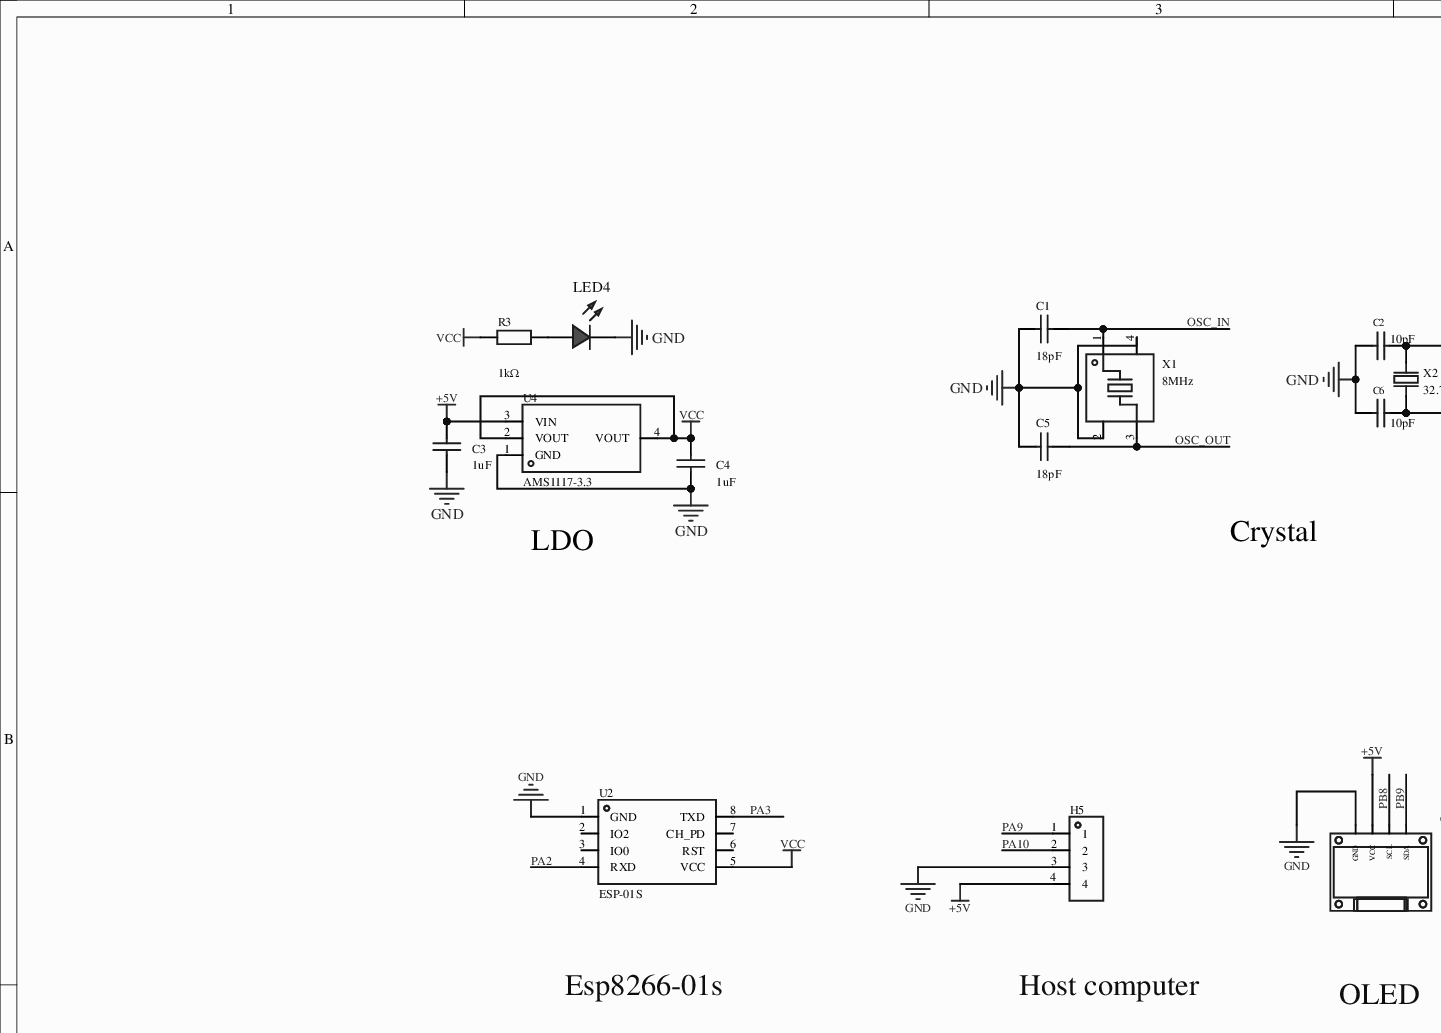
[diagram p0: MISC62726-3.schdoc, top left]
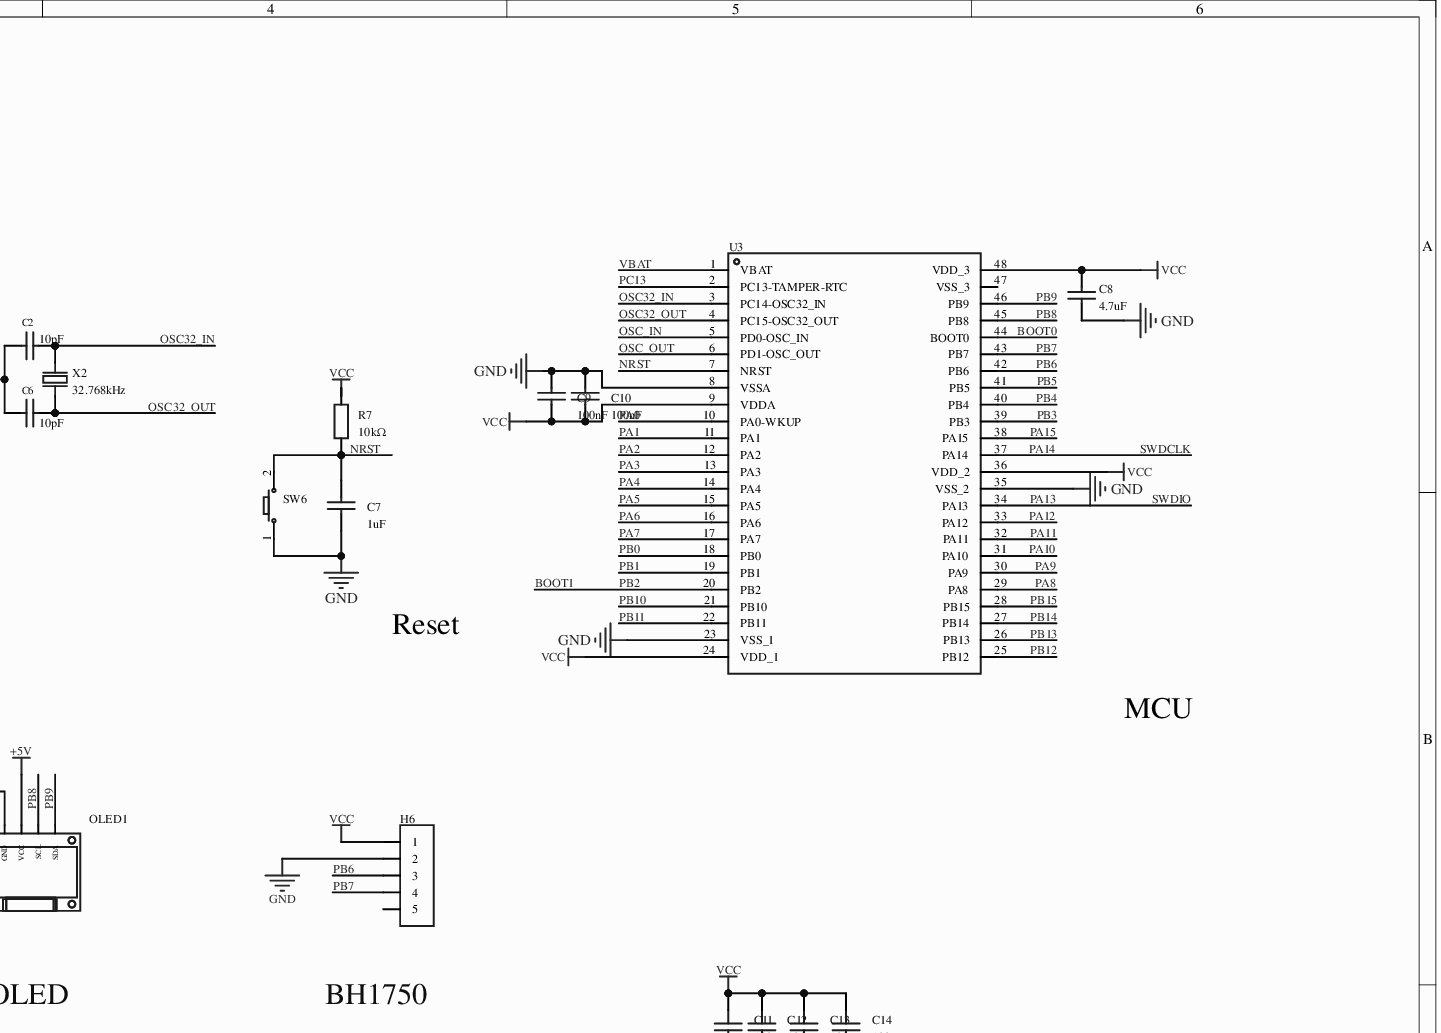
[diagram p1: MISC62726-3.schdoc, top right]
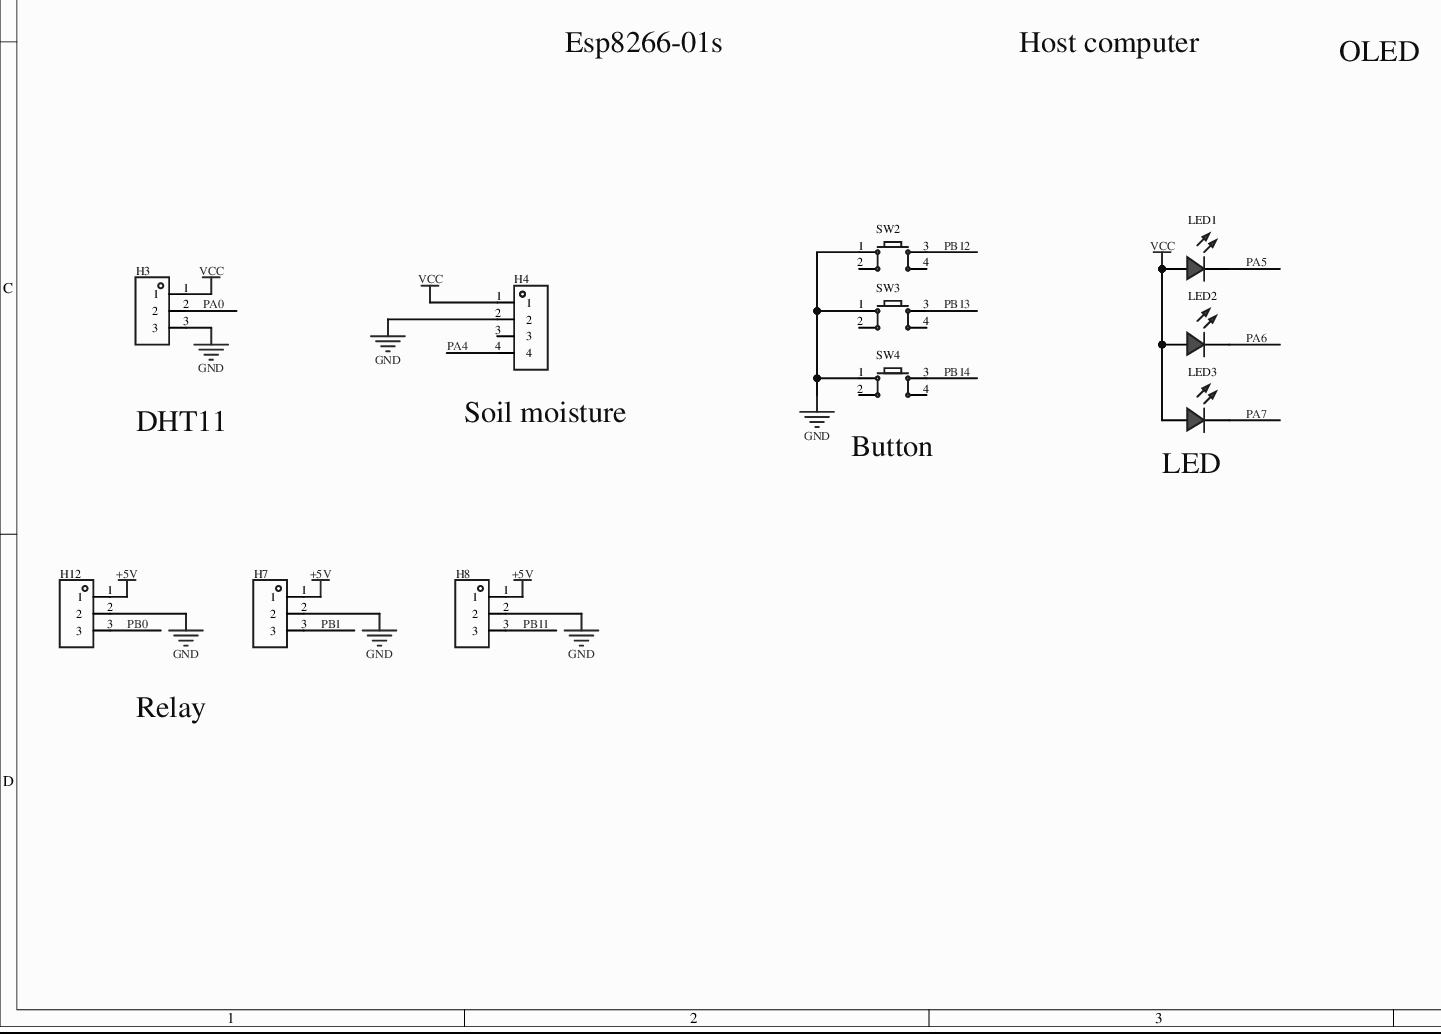
[diagram p2: MISC62726-3.schdoc, bottom left]
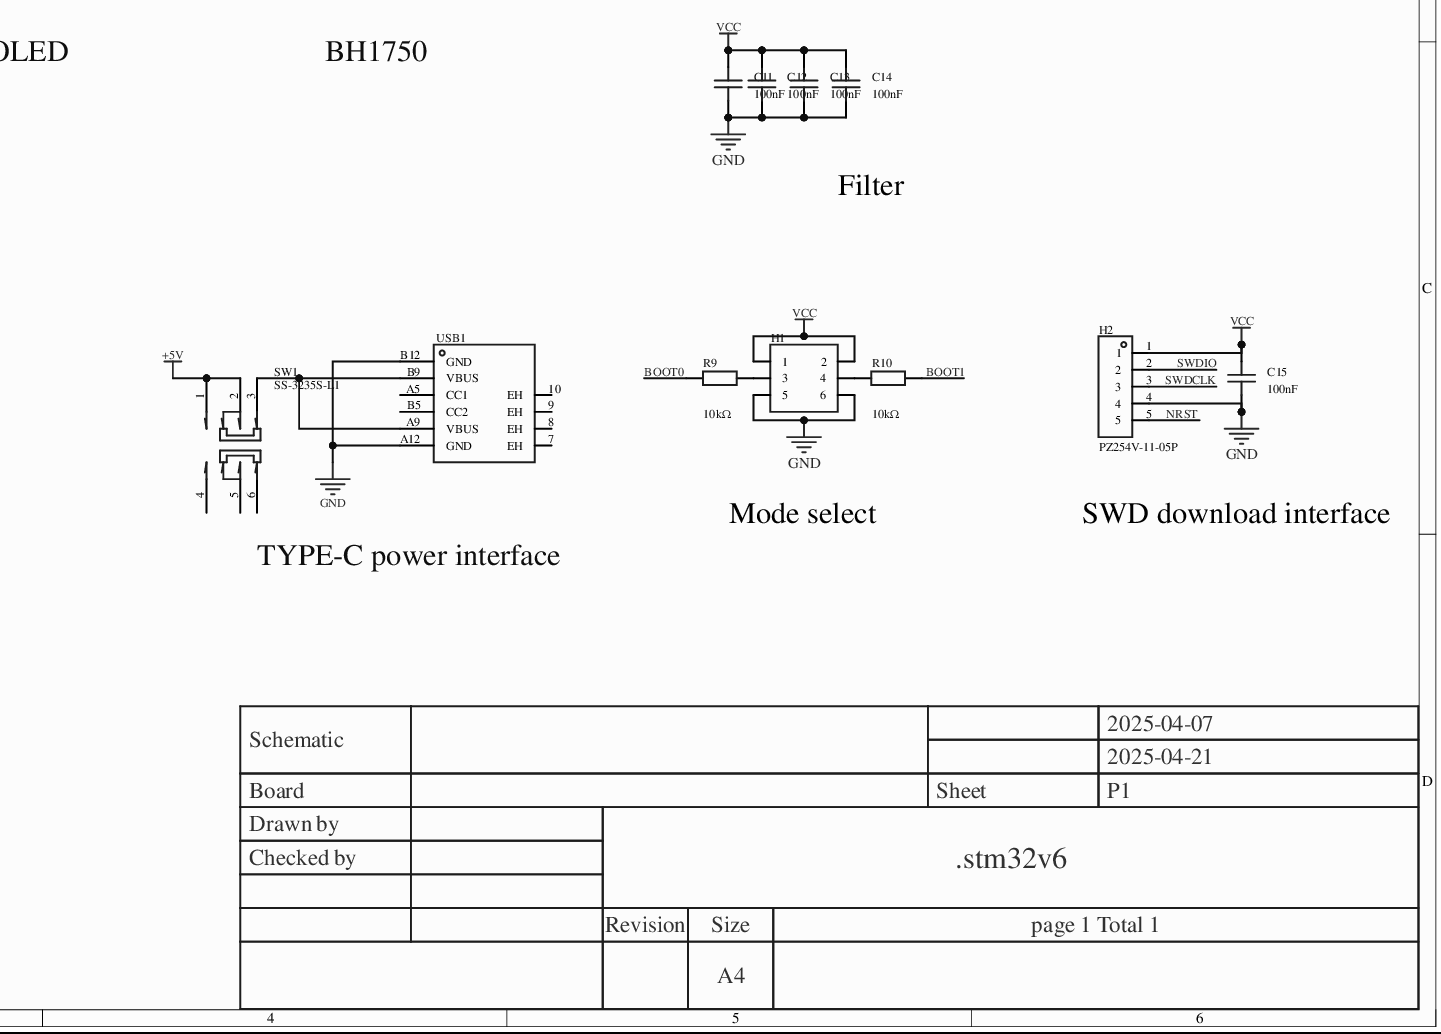
[diagram p3: MISC62726-3.schdoc, bottom right]
# Altium project MISC62726-2.PrjPcb
1 sheet, 44 parts. Net scope: global (net labels, ports and power ports of the same name join across sheets).
Board file: MISC62726.pcbdoc

## Sheet MISC62726-3.schdoc
size 420 x 297 mm; Version: V1.0; @Project Name: MISC62726; @Page Count: 1; @Update Date: 2026-04-13; @Create Date: 2026-04-13; @Schematic Name: MISC62726; @Page No: 1; @Create Time: 23:22:16; @Update Time: 17:32:40; @Board Name: MISC62726

### Parts
C1  18pF  [C0805]
C2  10pF  [C0805]
C3  1uF  [C0805]
C4  1uF  [C0805]
C5  18pF  [C0805]
C6  10pF  [C0805]
C7  1uF  [C0805]
C8  4.7uF  [C0805]
C9  100nF  [C0805]
C10  100nF  [C0805]
C11  100nF  [C0805]
C12  100nF  [C0805]
C13  100nF  [C0805]
C14  100nF  [C0805]
C15  100nF  [C0805]
H1  (no value)  [HDR-TH_6P-P2.54-V-R2-C3-S2.54_A2541WV-2X3P]
H2  PZ254V-11-05P  [HDR-TH_5P-P2.54-V-M]
H3  (no value)  [HDR-TH_3P-P2.54-V-F]
H4  (no value)  [HDR-TH_4P-P2.54-V-F]
H5  (no value)  [HDR-TH_4P-P2.54-V-F]
H6  (no value)  [HDR-TH_5P-P2.54-V-F]
H7  (no value)  [HDR-TH_3P-P2.54-V-F]
H8  (no value)  [HDR-TH_3P-P2.54-V-F]
H12  (no value)  [HDR-TH_3P-P2.54-V-F]
LED1  (no value)  [LED_TH-3mm]
LED2  (no value)  [LED_TH-3mm]
LED3  (no value)  [LED_TH-3mm]
LED4  (no value)  [LED_0402]
OLED1  (no value)  [0.96OLED_4P]
R3  1kΩ  [R0805]
R7  10kΩ  [R0805]
R9  10kΩ  [R0805]
R10  10kΩ  [R0805]
SW1  SS-3235S-L1  [SW-SMD_SS-3235S-LX]
SW2  (no value)  [SW-TH_4P-L6.0-W6.0-P4.50-LS6.5]
SW3  (no value)  [SW-TH_4P-L6.0-W6.0-P4.50-LS6.5]
SW4  (no value)  [SW-TH_4P-L6.0-W6.0-P4.50-LS6.5]
SW6  (no value)  [Key_SMD_3x4x2]
U2  ESP-01S  [WIFIM-TH_ESP-01S]
U3  STM32F103C8T6  [LQFP-48_L7.0-W7.0-P0.50-LS9.0-BL]  (value not drawn)
U4  AMS1117-3.3  [SOT-223-3_L6.5-W3.4-P2.30-LS7.0-BR]
USB1  (no value)  [USB_ TYPE-C-6P]
X1  8MHz  [OSC-SMD_4P-L3.2-W2.5-BL]
X2  32.768kHz  [CRYSTAL-SMD_L3.2-W1.5-1]

### Nets
+5V: C3.2 H5.4 H7.1 H8.1 H12.1 OLED1.2(VCC) SW1.1 SW1.2 U4.3(VIN)
GND: C1.2 C2.1 C3.1 C4.1 C5.2 C6.1 C7.2 C8.1 C9.2 C10.2 C11.1 C12.1 C13.1 C14.1 C15.1 H1.5 H1.6 H2.4 H3.3 H4.2 H5.3 H6.2 H7.2 H8.2 H12.2 LED4.1(C) OLED1.1(GND) SW2.1 SW3.1 SW4.1 SW6.1 U2.1(GND) U3.8(VSSA) U3.23(VSS_1) U3.35(VSS_2) U4.1(GND) USB1.A12(GND) USB1.B12(GND) X1.2(GND) X1.4(GND)
VCC: C4.2 C8.2 C9.1 C10.1 C11.2 C12.2 C13.2 C14.2 C15.2 H1.1 H1.2 H2.1 H3.1 H4.1 H6.1 LED1.1(C) LED2.1(C) LED3.1(C) R3.1 R7.2 U2.5(VCC) U3.9(VDDA) U3.24(VDD_1) U3.36(VDD_2) U3.48(VDD_3) U4.2(VOUT) U4.4(VOUT)
BOOT0: R9.1 U3.44(BOOT0)
BOOT1: R10.2 U3.20(PB2)  [also labelled PB2]
NRST: C7.1 H2.5 R7.1 SW6.2 U3.7(NRST)
OSC32_IN: C2.2 U3.3(PC14-OSC32_IN) X2.2
OSC32_OUT: C6.2 U3.4(PC15-OSC32_OUT) X2.1
OSC_IN: C1.1 U3.5(PD0-OSC_IN) X1.1
OSC_OUT: C5.1 U3.6(PD1-OSC_OUT) X1.3
PA0: H3.2 U3.10(PA0-WKUP)
PA1: U3.11(PA1)
PA2: U2.4(RXD) U3.12(PA2)
PA3: U2.8(TXD) U3.13(PA3)
PA4: H4.4 U3.14(PA4)
PA5: LED1.2(A) U3.15(PA5)
PA6: LED2.2(A) U3.16(PA6)
PA7: LED3.2(A) U3.17(PA7)
PA8: U3.29(PA8)
PA9: H5.1 U3.30(PA9)
PA10: H5.2 U3.31(PA10)
PA11: U3.32(PA11)
PA12: U3.33(PA12)
PA13: H2.2 U3.34(PA13)  [also labelled SWDIO]
PA14: H2.3 U3.37(PA14)  [also labelled SWDCLK]
PA15: U3.38(PA15)
PB0: H12.3 U3.18(PB0)
PB1: H7.3 U3.19(PB1)
PB3: U3.39(PB3)
PB4: U3.40(PB4)
PB5: U3.41(PB5)
PB6: H6.3 U3.42(PB6)
PB7: H6.4 U3.43(PB7)
PB8: OLED1.3(SCL) U3.45(PB8)
PB9: OLED1.4(SDA) U3.46(PB9)
PB10: U3.21(PB10)
PB11: H8.3 U3.22(PB11)
PB12: SW2.3 U3.25(PB12)
PB13: SW3.3 U3.26(PB13)
PB14: SW4.3 U3.27(PB14)
PB15: U3.28(PB15)
PC13: U3.2(PC13-TAMPER-RTC)
VBAT: U3.1(VBAT)
NetH1_3: H1.3 R9.2
NetH1_4: H1.4 R10.1
NetLED4_2: LED4.2(A) R3.2
NetSW1_3: SW1.3 USB1.A9(VBUS) USB1.B9(VBUS)

Not connected (* = marked no-connect by the designer): H4 3; H6 5; SW1 4 5 6; SW2 2 4; SW3 2 4; SW4 2 4; U2 2(IO2)* 3(IO0)* 6(RST)* 7(CH_PD)*; U3 47(VSS_3); USB1 7(EH) 8(EH) 9(EH) 10(EH) A5(CC1) B5(CC2)

### Notes on the sheet
- LDO
- Crystal
- Reset
- MCU
- Esp8266-01s
- Host computer
- OLED
- BH1750
- Filter
- DHT11
- (near H4) Soil moisture
- (near SW4) Button
- (near LED3) LED
- Mode select
- SWD download interface
- TYPE-C power interface
- Relay
- 2025-04-07
- Schematic
- Board
- Sheet
- 2025-04-21
- P1
- Drawn by
- Checked by
- .stm32v6
- Revision
- Size
- A4
- page 1 Total 1

### Library data of the parts
C1 C5 = FCC0603N180J500CT: Capacitance:18pF;Tolerance:±5%;Rated voltage:50V;Temperature coefficient:C0G;; Manufacturer: FOJAN(富捷); Symbol: 0402CG180J500NT; 3D Model: ac125912035d415993ca9572d50418b1; 3D Model Transform: 62.992,31.496,0,0,0,0,0,0,0; Tolerance: ±5%; Voltage Rating: 50V; Temperature Coefficient: C0G; AddInBom: yes; ModelName: C0603_L1.6-W0.8-H0.8; Device: FCC0603N180J500CT; Value: 18pF; LCSC Part Name: 18pF ±5% 50V; Supplier Footprint: 0603; Datasheet: https://atta.szlcsc.com/upload/public/pdf/source/20220818/0EB3B7FB2F5648AC16609637FBA7DABE.pdf; Supplier: LCSC; Manufacturer Part: FCC0603N180J500CT; Supplier Part: C5137620; JLCPCB Part Class: Extended Part; ConvertToPcb: yes; FootprintName: C0805
C2 C6 = CL10C100JB8NNNC: Capacitance:10pF;Tolerance:±5%;Rated voltage:50V;Temperature coefficient:C0G;; Manufacturer: SAMSUNG(三星); Symbol: 0402CG100J500NT; 3D Model: ac125912035d415993ca9572d50418b1; 3D Model Transform: 62.992,31.496,0,0,0,0,0,0,0; Tolerance: ±5%; Voltage Rating: 50V; Temperature Coefficient: C0G; AddInBom: yes; ModelName: C0603_L1.6-W0.8-H0.8; Device: CL10C100JB8NNNC; Value: 10pF; LCSC Part Name: 10pF ±5% 50V; Supplier Footprint: 0603; Datasheet: https://item.szlcsc.com/datasheet/CL10C100JB8NNNC/1986.html; Supplier: LCSC; Manufacturer Part: CL10C100JB8NNNC; Capacitance: 10pF; Supplier Part: C1634; JLCPCB Part Class: Basic Part; ConvertToPcb: yes; FootprintName: C0805
C3 = CL05A105KP5NNNC: Capacitance:1uF;Tolerance:±10%;Rated voltage:10V;Dielectric (temperature coefficient):X5R;; Manufacturer: SAMSUNG(三星); 3D Model: 36a51122f27c49738f86b3bfa98863e0; 3D Model Transform: 39.37,19.685,0,0,0,0,0,0,0; Tolerance: ±10%; Voltage Rated: 10V; Temperature Coefficient: X5R; AddInBom: yes; ModelName: C0402_L1.0-W0.5-H0.5; Symbol: CL05A105KP5NNNC; Device: CL05A105KP5NNNC; Value: 1uF; LCSC Part Name: 1uF ±10% 10V; Supplier Footprint: 0402; Datasheet: https://atta.szlcsc.com/upload/public/pdf/source/20160218/1457707763339.pdf; Supplier: LCSC; Manufacturer Part: CL05A105KP5NNNC; Supplier Part: C14445; JLCPCB Part Class: Extended Part; ConvertToPcb: yes; FootprintName: C0805
C4 = CL05A105KQ5NNNC: Capacitance:1uF;Tolerance:±10%;Rated voltage:6.3V;Dielectric (temperature coefficient):X5R;; Manufacturer: SAMSUNG(三星); 3D Model: 36a51122f27c49738f86b3bfa98863e0; 3D Model Transform: 39.37,19.685,0,0,0,0,0,0,0; Tolerance: ±10%; Voltage Rated: 6.3V; Temperature Coefficient: X5R; AddInBom: yes; ModelName: C0402_L1.0-W0.5-H0.5; Symbol: CL05A105KQ5NNNC; Device: CL05A105KQ5NNNC; Value: 1uF; LCSC Part Name: 1uF ±10% 6.3V; Supplier Footprint: 0402; Datasheet: https://atta.szlcsc.com/upload/public/pdf/source/20160218/1457707763339.pdf; Supplier: LCSC; Manufacturer Part: CL05A105KQ5NNNC; Supplier Part: C107372; JLCPCB Part Class: Extended Part; ConvertToPcb: yes; FootprintName: C0805
C7 = CGA0603X5R105K500JT: Capacitance:1uF;Tolerance:±10%;Rated voltage:50V;Temperature coefficient:X5R;; Manufacturer: HRE(芯声); Symbol: CL05A105KQ5NNNC; 3D Model: ac125912035d415993ca9572d50418b1; 3D Model Transform: 62.992,31.496,0,0,0,0,0,0,0; Tolerance: ±10%; Voltage Rating: 50V; Temperature Coefficient: X5R; AddInBom: yes; ModelName: C0603_L1.6-W0.8-H0.8; Device: CGA0603X5R105K500JT; Value: 1uF; LCSC Part Name: 1uF ±10% 50V; Supplier Footprint: 0603; Supplier: LCSC; Manufacturer Part: CGA0603X5R105K500JT; Supplier Part: C6119852; JLCPCB Part Class: Extended Part; ConvertToPcb: yes; FootprintName: C0805
C8 = CL10A475KO8NNNC: Capacitance:4.7uF;Tolerance:±10%;Rated voltage:16V;Temperature coefficient:X5R;; Manufacturer: SAMSUNG(三星); Symbol: CL05A475MP5NRNC; 3D Model: ac125912035d415993ca9572d50418b1; 3D Model Transform: 62.992,31.496,0,0,0,0,0,0,0; Tolerance: ±10%; Voltage Rating: 16V; Temperature Coefficient: X5R; AddInBom: yes; ModelName: C0603_L1.6-W0.8-H0.8; Device: CL10A475KO8NNNC; Value: 4.7uF; LCSC Part Name: 4.7uF ±10% 16V; Supplier Footprint: 0603; Datasheet: https://item.szlcsc.com/datasheet/CL10A475KO8NNNC/20375.html; Supplier: LCSC; Manufacturer Part: CL10A475KO8NNNC; Supplier Part: C19666; JLCPCB Part Class: Basic Part; ConvertToPcb: yes; FootprintName: C0805
C9 = CC0603KRX7R9BB104: Capacitance:100nF;Tolerance:±10%;Rated voltage:50V;Temperature coefficient:X7R;; Manufacturer: YAGEO(国巨); Symbol: CC0402KRX7R9BB103; 3D Model: ac125912035d415993ca9572d50418b1; 3D Model Transform: 62.992,31.496,0,0,0,0,0,0,0; Tolerance: ±10%; Voltage Rating: 50V; Temperature Coefficient: X7R; AddInBom: yes; ModelName: C0603_L1.6-W0.8-H0.8; Device: CC0603KRX7R9BB104; Value: 100nF; LCSC Part Name: 100nF ±10% 50V; Supplier Footprint: 0603; Datasheet: https://item.szlcsc.com/datasheet/CC0603KRX7R9BB104/15331.html; Supplier: LCSC; Manufacturer Part: CC0603KRX7R9BB104; Supplier Part: C14663; JLCPCB Part Class: Basic Part; ConvertToPcb: yes; FootprintName: C0805
C10 = CC0603KRX7R9BB104: Capacitance:100nF;Tolerance:±10%;Rated voltage:50V;Temperature coefficient:X7R;; Manufacturer: YAGEO(国巨); Symbol: CL05A105KP5NNNC; 3D Model: ac125912035d415993ca9572d50418b1; 3D Model Transform: 62.992,31.496,0,0,0,0,0,0,0; Tolerance: ±10%; Voltage Rating: 50V; Temperature Coefficient: X7R; AddInBom: yes; ModelName: C0603_L1.6-W0.8-H0.8; Device: CC0603KRX7R9BB104; Value: 100nF; LCSC Part Name: 100nF ±10% 50V; Supplier Footprint: 0603; Datasheet: https://item.szlcsc.com/datasheet/CC0603KRX7R9BB104/15331.html; Supplier: LCSC; Manufacturer Part: CC0603KRX7R9BB104; Supplier Part: C14663; JLCPCB Part Class: Basic Part; ConvertToPcb: yes; FootprintName: C0805
C11-C15 = CC0603KRX7R9BB104: Capacitance:100nF;Tolerance:±10%;Rated voltage:50V;Temperature coefficient:X7R;; Manufacturer: YAGEO(国巨); Symbol: CC0402KRX7R7BB104; 3D Model: ac125912035d415993ca9572d50418b1; 3D Model Transform: 62.992,31.496,0,0,0,0,0,0,0; Tolerance: ±10%; Voltage Rating: 50V; Temperature Coefficient: X7R; AddInBom: yes; ModelName: C0603_L1.6-W0.8-H0.8; Device: CC0603KRX7R9BB104; Value: 100nF; LCSC Part Name: 100nF ±10% 50V; Supplier Footprint: 0603; Datasheet: https://item.szlcsc.com/datasheet/CC0603KRX7R9BB104/15331.html; Supplier: LCSC; Manufacturer Part: CC0603KRX7R9BB104; Supplier Part: C14663; JLCPCB Part Class: Basic Part; ConvertToPcb: yes; FootprintName: C0805
H1 = HDR-M_2.54_2x3: Symbol: HDR-M-2.54_2x3; 3D Model: fd1b55b786fb415ca65c4187088147b7; 3D Model Transform: 299.9994,200,0,0,0,0,0,0,-118.11; ConvertToPcb: yes; ModelName: HDR2.54-M-LI-2x3P; Device: HDR-M_2.54_2x3; Supplier Part: C402781; Supplier Footprint: 插件,P=2.54mm; AddInBom: yes; FootprintName: HDR-TH_6P-P2.54-V-R2-C3-S2.54_A2541WV-2X3P
H2 = PZ254V-11-05P: Pin structure:1x5P;Pitch:2.54mm;Row pitch:-;Round/square pin:Square pin;Mounting:Through-hole;Rows:Single row;Total pins:5P;Rated current:-;Rated voltage:-;Mating pin length:6mm;Insulator height:2.5mm;Tail length:3mm;Contact material:Brass;Contact plating:-;Operating temperature:-40℃~+105℃;Colour:Black;; Manufacturer: XFCN(兴飞); 3D Model: 47d466e4a34f4fc5bc626cf773a24dd5; 3D Model Transform: 499.999,100,0,0,0,0,0,0,-118.11; Pin Structure: 1x5P; Pitch: 2.54mm; Circluar Pins/Square Pins: Square; AddInBom: yes; ModelName: HDR-TH_5P-P2.54-M-LI-1X5P; Symbol: PZ254V-11-05P; Device: PZ254V-11-05P; LCSC Part Name: 1x5P 间距:2.54mm 方针 直插; Supplier Part: C492404; Manufacturer Part: PZ254V-11-05P; Supplier Footprint: 插件,P=2.54mm; JLCPCB Part Class: Extended Part; Datasheet: https://atta.szlcsc.com/upload/public/pdf/source/20200309/C492404_E51533260F8710EFF5D4617281164C1D.pdf; Supplier: LCSC; Row Spacing: -; Mounting Type: Through-hole; Number of Rows: Single row; Number of Pins: 5P; Current Rating: -; Voltage Rating (Max): -; Length of Mating Pin: 6mm; Insulation Height: 2.5mm; Length of End Connection Pin: 3mm; Contact Material: Brass; Contact Plating: -; Operating Temperature: -40℃~+105℃; Color: Black; ConvertToPcb: yes; FootprintName: HDR-TH_5P-P2.54-V-M
H3 H7 H8 H12 = HDR-F_2.54_1x3P: Symbol: PM254V-11-03-H85; 3D Model: f3b3cc5aae9641bf9e56fc160cef875b; 3D Model Transform: 299.9994,100,0,0,0,0,0,0,-118.11; ConvertToPcb: yes; ModelName: HDR2.54-F-LI-1X3P; Device: HDR-F_2.54_1x3P; Supplier Part: C541850; Supplier Footprint: 插件; FootprintName: HDR-TH_3P-P2.54-V-F; AddInBom: yes
H4 = HDR-F_2.54_1x4P: Symbol: 2.54-1*4P female; ConvertToPcb: yes; ModelId: d187812051054f85879fcaa51a310d8e0819f05c4eef4c71ace90d822a990e87; ModelTransform: 419.6842,98.464,0,0,0,0,0,0,-118.11; Device: HDR-F_2.54_1x4P; FootprintName: HDR-TH_4P-P2.54-V-F; AddInBom: yes; SupplierPart: C2718488; Supplier Footprint: 插件; ModelName: HDR-TH_4P-P2.54-V-F
H5 = HDR-F_2.54_1x4P: Symbol: 2.54-1*4P female; 3D Model: d187812051054f85879fcaa51a310d8e0819f05c4eef4c71ace90d822a990e87; 3D Model Transform: 419.6842,98.464,0,0,0,0,0,0,-118.11; ConvertToPcb: yes; Device: HDR-F_2.54_1x4P; Supplier Part: C2718488; Supplier Footprint: 插件; FootprintName: HDR-TH_4P-P2.54-V-F; AddInBom: yes; ModelName: HDR-TH_4P-P2.54-V-F
H6 = HDR-F_2.54_1x5P: Symbol: Header-Female-2.54_1x5; ConvertToPcb: yes; ModelId: f49cb6116a3d45e5a64915bf3e00773f; ModelTransform: 519.684,98.464,0,0,0,0,0,0,-124.016; Device: HDR-F_2.54_1x5P; AddInBom: yes; SupplierPart: C50950; Supplier Footprint: 插件; FootprintName: HDR-TH_5P-P2.54-V-F; ModelName: HDR-TH_5P-P2.54-V-F
LED1-LED3 = LED_TH-R_3mm: ConvertToPcb: yes; ModelId: a497c992633541038a38947cdc58012f0819f05c4eef4c71ace90d822a990e87; ModelName: LED-TH-3mm_R; ModelTransform: 141.274,153.327,0,0,0,0,-5.984,0,-137.795; Symbol: LED_TH-R; Device: LED_TH-R_3mm; AddInBom: yes; FootprintName: LED_TH-3mm; Supplier Footprint: 插件
LED4 = LED_0402-R: Symbol: LED_R; Convert to PCB: yes; 3D Model: ff479c6f784e45d5abe8f8ff531b4a70; 3D Model Transform: 39.4,19.7,15.76,180,0,0,0,0,0; ModelName: LED0402-RD_ORANGE; Device: LED_0402-R; Add into BOM: yes; Supplier Footprint: 0402; FootprintName: LED_0402
OLED1 = 0.96OLED模块_4P: ConvertToPcb: yes; ModelId: 79c000fdb68d45a296c2e9bedf4f9055; ModelTransform: 1393.69792,1318.895,0,0,0,0,0,-560.079,-137.795; Device: 0.96OLED模块_4P; Symbol: 0.96OLED模块_4P; FootprintName: 0.96OLED_4P; AddInBom: yes; Supplier Footprint: 插件; ModelName: 0.96OLED_4P
R3 = 0603WAF1001T5E: Resistor type:Thick film resistor;Resistance:1kΩ;Tolerance:±1%;Power:100mW;Max operating voltage:75V;Temperature coefficient:±100ppm/℃;; Manufacturer: UNI-ROYAL(厚声); Symbol: 0402WGF1001TCE; 3D Model: fc143cca1e79419f9cd78b61e9279f08; 3D Model Transform: 31.8897,63.7794,0,90,0,0,0,0,0; Tolerance: ±1%; Power(Watts): 100mW; Overload Voltage (Max): 75V; AddInBom: yes; ModelName: R0603; Device: 0603WAF1001T5E; Value: 1kΩ; JLCPCB Part Class: Basic Part; LCSC Part Name: 1kΩ ±1% 100mW 厚膜电阻; Supplier Footprint: 0603; Datasheet: https://atta.szlcsc.com/upload/public/pdf/source/20200306/C422600_1E6D84923E4A46A82E41ADD87F860B5C.pdf; Type: Thick film resistor; Temperature Coefficient: ±100ppm/℃; Operating Temperature Range: -55℃~+155℃; Supplier: LCSC; Manufacturer Part: 0603WAF1001T5E; Supplier Part: C21190; ConvertToPcb: yes; FootprintName: R0805
R7 R9 R10 = 0603WAF1002T5E: Resistor type:Thick film resistor;Resistance:10kΩ;Tolerance:±1%;Power:100mW;Operating voltage:75V;Temperature coefficient:±100ppm/℃;; Manufacturer: UNI-ROYAL(厚声); Symbol: RC0402FR-0710KL; 3D Model: fc143cca1e79419f9cd78b61e9279f08; 3D Model Transform: 31.8897,63.7794,0,90,0,0,0,0,0; Tolerance: ±1%; Power(Watts): 100mW; Voltage-Supply(Max): 75V; AddInBom: yes; ModelName: R0603; Device: 0603WAF1002T5E; Value: 10kΩ; LCSC Part Name: 厚膜电阻 10kΩ ±1% 100mW; Supplier Part: C25804; Manufacturer Part: 0603WAF1002T5E; Supplier Footprint: 0603; JLCPCB Part Class: Basic Part; Datasheet: https://item.szlcsc.com/datasheet/0603WAF1002T5E/26547.html; Supplier: LCSC; Type: Thick film resistor; Temperature Coefficient: ±100ppm/℃; Operating Temperature: -55℃~+155℃; Overload Voltage (Max): 75V; Operating Temperature Range: -55℃~+155℃; ConvertToPcb: yes; FootprintName: R0805
SW1 = SS-3235S-L1: Circuit structure:DPDT;Mounting:Horizontal SMD;Switch colour:Black;Rated current:50mA;Rated voltage:12V;Operating life:1 ten-thousand cycles;; Manufacturer: XKB Connection(中国星坤); AddInBom: yes; ModelId: e98810a9d4c646b4962907642f59f8260819f05c4eef4c71ace90d822a990e87; ModelTransform: 356.299,271.653,0,0,0,0,0.002,-0.004,0; Circuit: DPDT; Actuator Style: Rectangular column; Switch Height: 3.2mm; Actuator Color: Black; Current Rating: 50mA; Voltage Rating: 12V; Symbol: SS-3235S-L1; Device: SS-3235S-L1; LCSC Part Name: 柄长2mm 卧贴双档 滑动开关; SupplierPart: C500055; ManufacturerPart: SS-3235S-L1; Supplier Footprint: SMD,9.1x3.6mm; JLCPCB Part Class: Extended Part; Datasheet: https://item.szlcsc.com/datasheet/SS-3235S-L1/512181.html; Supplier: LCSC; ConvertToPcb: yes; FootprintName: SW-SMD_SS-3235S-LX; ModelName: SW-SMD_SS-3235S-LX; Termination Style: Gull-wing; Length: 9.1mm; Width: 3.55mm; Mounting Type: Horizontal SMD; Life: 1 ten-thousand cycles; Operating Temperature: -40℃~+85℃
SW2-SW4 = Key_TH_6x6x6: Contact current:50mA;Rated voltage(DC):12V;Insulation resistance:100MΩ;Circuit structure:SPST;Mounting:Through-hole;Button shape:Round button;Button/cap colour:Black;Actuation force:260gf@±30gf;Operating temperature:-25℃~+70℃;Pin style:PC pin;Switch length:6mm;Switch width:6mm;Switch height:6mm;With bracket:No;; Symbol: Tact switch; AddInBom: yes; ModelId: 20eee248bc684ccd8cbdbb1d0d91ec6f0819f05c4eef4c71ace90d822a990e87; ModelName: SW-TH_4P-L6.0-W6.0-H5.0-LS6.5-P4.50; ModelTransform: 236.22,323.03,0,90,0,0,0,0,-137.795; Device: Key_TH_6x6x6; FootprintName: SW-TH_4P-L6.0-W6.0-P4.50-LS6.5; ConvertToPcb: yes; Supplier Footprint: 插件
SW6 = Key_SMD_3x4x2: Symbol: Tact switch x2; ConvertToPcb: yes; ModelId: 63599cce708d48afbce1b0db003544770819f05c4eef4c71ace90d822a990e87; ModelName: SW-SMD_L4.0-W2.9-H2-LS5.0; ModelTransform: 196.85,114.17,79.13,0,0,0,0,0,0; Device: Key_SMD_3x4x2; AddInBom: yes; Supplier Footprint: SMD; FootprintName: Key_SMD_3x4x2
U2 = ESP-01S_C111009: 3D Model: eb7175da78ae48b3b1568cfe3027405f0819f05c4eef4c71ace90d822a990e87; 3D Model Transform: 582.676,976.37608,0,0,0,0,0,388.346,-118.11; AddInBom: yes; Symbol: ESP-01S; Device: ESP-01S_C111009; LCSC Part Name: ESP-01S; Supplier Part: C111009; Manufacturer Part: ESP-01S; Supplier Footprint: -; JLCPCB Part Class: Extended Part; Supplier: LCSC; ConvertToPcb: yes; FootprintName: WIFIM-TH_ESP-01S; ModelName: WIFIM-TH_ESP-01S
U3 = STM32F103C8T6: CPU core:CM3;Program memory capacity:64KB;Total RAM:20KB;GPIO count:37;Operating voltage range:2V~3.6V;Max CPU frequency:72MHz;Program memory type:FLASH;; Manufacturer: ST(意法半导体); 3D Model: 093be70396ff421eb2cdb946d5311efc; 3D Model Transform: 354.331,354.331,0,0,0,0,0,0,0; CPU Core: CM3; Program Storage Size: 64KB; RAM Size: 20KB; GPIO Ports Number: 37; CPU Maximum Speed: 72MHz; Program Memory Type: FLASH; ADC (Bit): 12bit; Universal Serial Bus: Yes; Peripheral/Function: Watchdog; DMA; Watchdog; On-chip temperature sensor; ModelName: LQFP-48_L7.0-W7.0-H1.4-LS9.0-P0.50; Symbol: STM32F103C8T6; Device: STM32F103C8T6; LCSC Part Name: STM32F103C8T6 MSL=3; Supplier Part: C8734; Manufacturer Part: STM32F103C8T6; Supplier Footprint: LQFP-48(7x7); JLCPCB Part Class: Extended Part; Datasheet: https://atta.szlcsc.com/upload/public/pdf/source/20220812/8363ACEC51AD55ECEB84799464F7CB85.pdf; Supplier: LCSC; Operating Voltage Range: 2V~3.6V; Operating Temperature Range: -40℃~+85℃; DAC (Bit): -; PWM (Bit): -; Internal Comparator: -; communication protocol: -; Watchdog: Yes; Real-Time Clock: -; Infrared Data Association: Yes; Low-Voltage Detect: Yes; CCP Capture/Compare: -; Secure Digital Input and Output: -; Direct Memory Access: Yes; Internal Oscillator: Yes; AddInBom: yes; ConvertToPcb: yes; FootprintName: LQFP-48_L7.0-W7.0-P0.50-LS9.0-BL
U4 = AMS1117-3.3_C6186: Output type:Fixed;Operating voltage:-;Output voltage:3.3V;Output current:1A;Power supply rejection ratio (PSRR):72dB@(120Hz);Output polarity:Positive;; Manufacturer: AMS; AddInBom: yes; ModelId: 925194bf9823436183a3e0b978a8d076; ModelName: SOT-223-4P_L6.5-W3.5-H1.6-LS7.0-P2.30; ModelTransform: 279.89794,255.905,0,180,0,0,-3.9385,-0.0005,0; Output Type: Fixed; Output Voltage: 3.3V; Output Current: 1A; Voltage Dropout: 1.3V@(800mA); Number of Outputs: 1; Symbol: AMS1117-3.3; Device: AMS1117-3.3_C6186; LCSC Part Name: 输出3.3V 1A; SupplierPart: C6186; ManufacturerPart: AMS1117-3.3; Supplier Footprint: SOT-223; Datasheet: https://atta.szlcsc.com/upload/public/pdf/source/20180727/C6186_7A095716F0823C02F1997A905E26C086.pdf; Supplier: LCSC; ConvertToPcb: yes; FootprintName: SOT-223-3_L6.5-W3.4-P2.30-LS7.0-BR; Voltage - Supply: -; Power Supply Rejection Ratio (PSRR): 72dB@(120Hz); standby current: -; Noise: -; Features: Overcurrent protection (OCP); Thermal shutdown (TSD); Operating Temperature: -; Output Configuration: Positive
USB1 = USB_ Type-C-6P: AddInBom: yes; ModelId: d4f492a4e6024845a13b3f6a4ef2d2cb0819f05c4eef4c71ace90d822a990e87; ModelName: USB-SMD_U262-061N-4BVC11; ModelTransform: 352.362,281.496,0,0,0,0,0,-47.244,-39.37; Symbol: USB_ TYPE-C-6P; Device: USB_ Type-C-6P; Supplier Footprint: SMD; ConvertToPcb: yes; FootprintName: USB_ TYPE-C-6P
X1 = X32258MOB4SI: Crystal type:SMD crystal;Frequency:8MHz;Frequency tolerance (ambient):±10ppm;Load capacitance:12pF;Frequency stability (full temp.):±20ppm;; Manufacturer: YXC(扬兴晶振); 3D Model: ae22b8d143894765bc8100c37cb6356f; 3D Model Transform: 125.984,98.425,0,0,0,0,0,0,0; Normal temperature Frequency Tolerance: ±10ppm; External load capacitor: 12pF; Frequency Stability(Full temperature range): ±20ppm; Equivalent Series Resistance (ESR): 150Ω; AddInBom: yes; ModelName: OSC-SMD_4P-L3.2-W2.5-H1.0; Symbol: X32258MOB4SI; Device: X32258MOB4SI; LCSC Part Name: 8MHz ±10ppm 12pF; Supplier Part: C2682775; Manufacturer Part: X32258MOB4SI; Supplier Footprint: SMD3225-4P; JLCPCB Part Class: Extended Part; Datasheet: https://atta.szlcsc.com/upload/public/pdf/source/20240329/19D5F850207469550BEB00D7DFEDBC7A.pdf; Supplier: LCSC; Crystal Type: SMD crystal; Value: 8MHz; Operating Temperature: -40℃~+85℃; ConvertToPcb: yes; FootprintName: OSC-SMD_4P-L3.2-W2.5-BL
X2 = Q13FC13500049: Crystal type:SMD crystal;Frequency:32.768kHz;Frequency tolerance (ambient):±20ppm;Load capacitance:6pF;; Manufacturer: EPSON(爱普生); Symbol: Q13FC1350004900; 3D Model: 762d7afc596f4558a373612390f4386d; 3D Model Transform: 125.984,59.055,0,0,0,0,0,0,0; Normal temperature Frequency Tolerance: ±20ppm; External load capacitor: 6pF; Equivalent Series Resistance (ESR): 70kΩ; AddInBom: yes; Device: Q13FC13500049; Value: 32.768kHz; LCSC Part Name: 32.768kHz ±20ppm 6pF; Supplier Part: C95361; Manufacturer Part: Q13FC13500049; Supplier Footprint: SMD3215-2P; JLCPCB Part Class: Extended Part; Datasheet: https://atta.szlcsc.com/upload/public/pdf/source/20230307/B34DAB909D91A4E9CF7EB9FB947CF9CB.pdf; Supplier: LCSC; Crystal Type: SMD crystal; Operating Temperature: -40℃~+85℃; ConvertToPcb: yes; FootprintName: CRYSTAL-SMD_L3.2-W1.5-1; ModelName: CRYSTAL-SMD_L3.2-W1.5-1